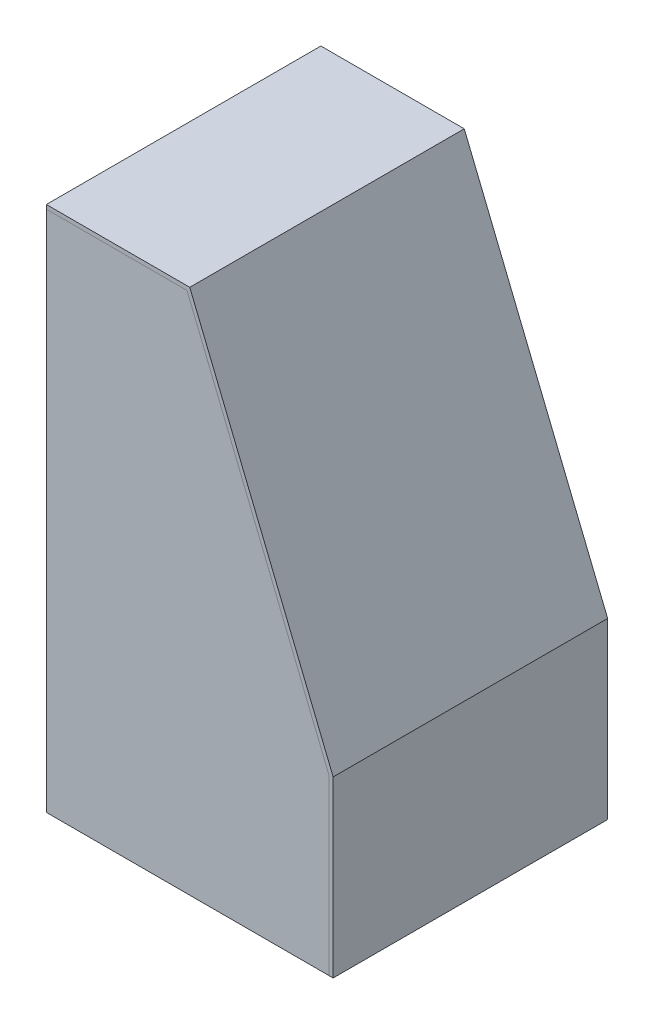
from build123d import *

# Parameters (mm, degrees)
EXTRUDE_1_DEPTH   = 134
EXTRUDE_1_2_DEPTH = 2
EXTRUDE_START     = -134
EXTRUDE_2_DEPTH   = 2


with BuildPart() as part:
    # 草图1 → Extrude 1 (new body)
    with BuildSketch(Plane.XY):
        Polygon((0, 0), (70, 0), (140, -172), (140, -257), (138, -257), (138, -172.391390876), (68.654666504, -2), (0, -2), align=None)
    extrude(amount=EXTRUDE_1_DEPTH)


with BuildPart() as body_2:
    # 草图2 → Extrude 1 2 (new body)
    with BuildSketch(Plane.XY.offset(134)):
        Polygon((0, -2), (68.654666504, -2), (138, -172.391390876), (138, -257), (0, -257), align=None)
    extrude(amount=-EXTRUDE_1_2_DEPTH)


with BuildPart() as body_3:
    # 草图2<2> → 凸台-拉伸2 (new body)
    with BuildSketch(Plane.XY.offset(134).offset(EXTRUDE_START)):
        Polygon((0, -2), (68.654666504, -2), (138, -172.391390876), (138, -257), (0, -257), align=None)
    extrude(amount=EXTRUDE_2_DEPTH)


solid = Compound([part.part, body_2.part, body_3.part])
